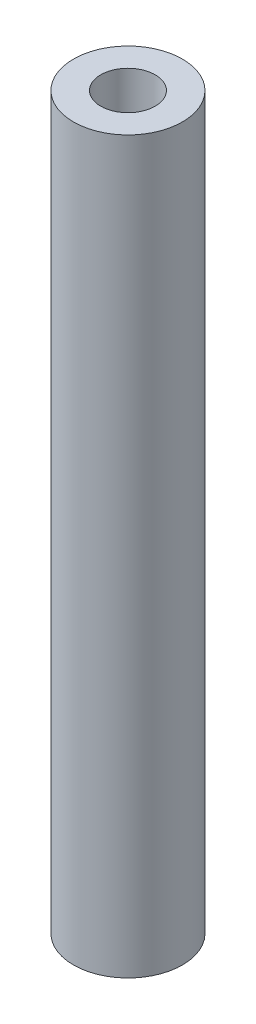
SolidWorks part; units mm, degrees
material "ABS"
ref_plane "Front Plane" through (0, 0, 0) normal (0, 0, 1) x (1, 0, 0)
ref_plane "Top Plane" through (0, 0, 0) normal (0, 1, 0) x (1, 0, 0)
ref_plane "Right Plane" through (0, 0, 0) normal (1, 0, 0) x (0, 0, -1)
sketch "Sketch1" plane through (0, 0, 0) normal (0, 1, 0) x (1, 0, 0)
  circle A0 centre (0, 0) radius 1
  circle A1 centre (0, 0) radius 0.5
  dimension "D1" = 2
  dimension "D2" = 1
extrude "Boss-Extrude1" add sketch "Sketch1" along normal blind 13.4
